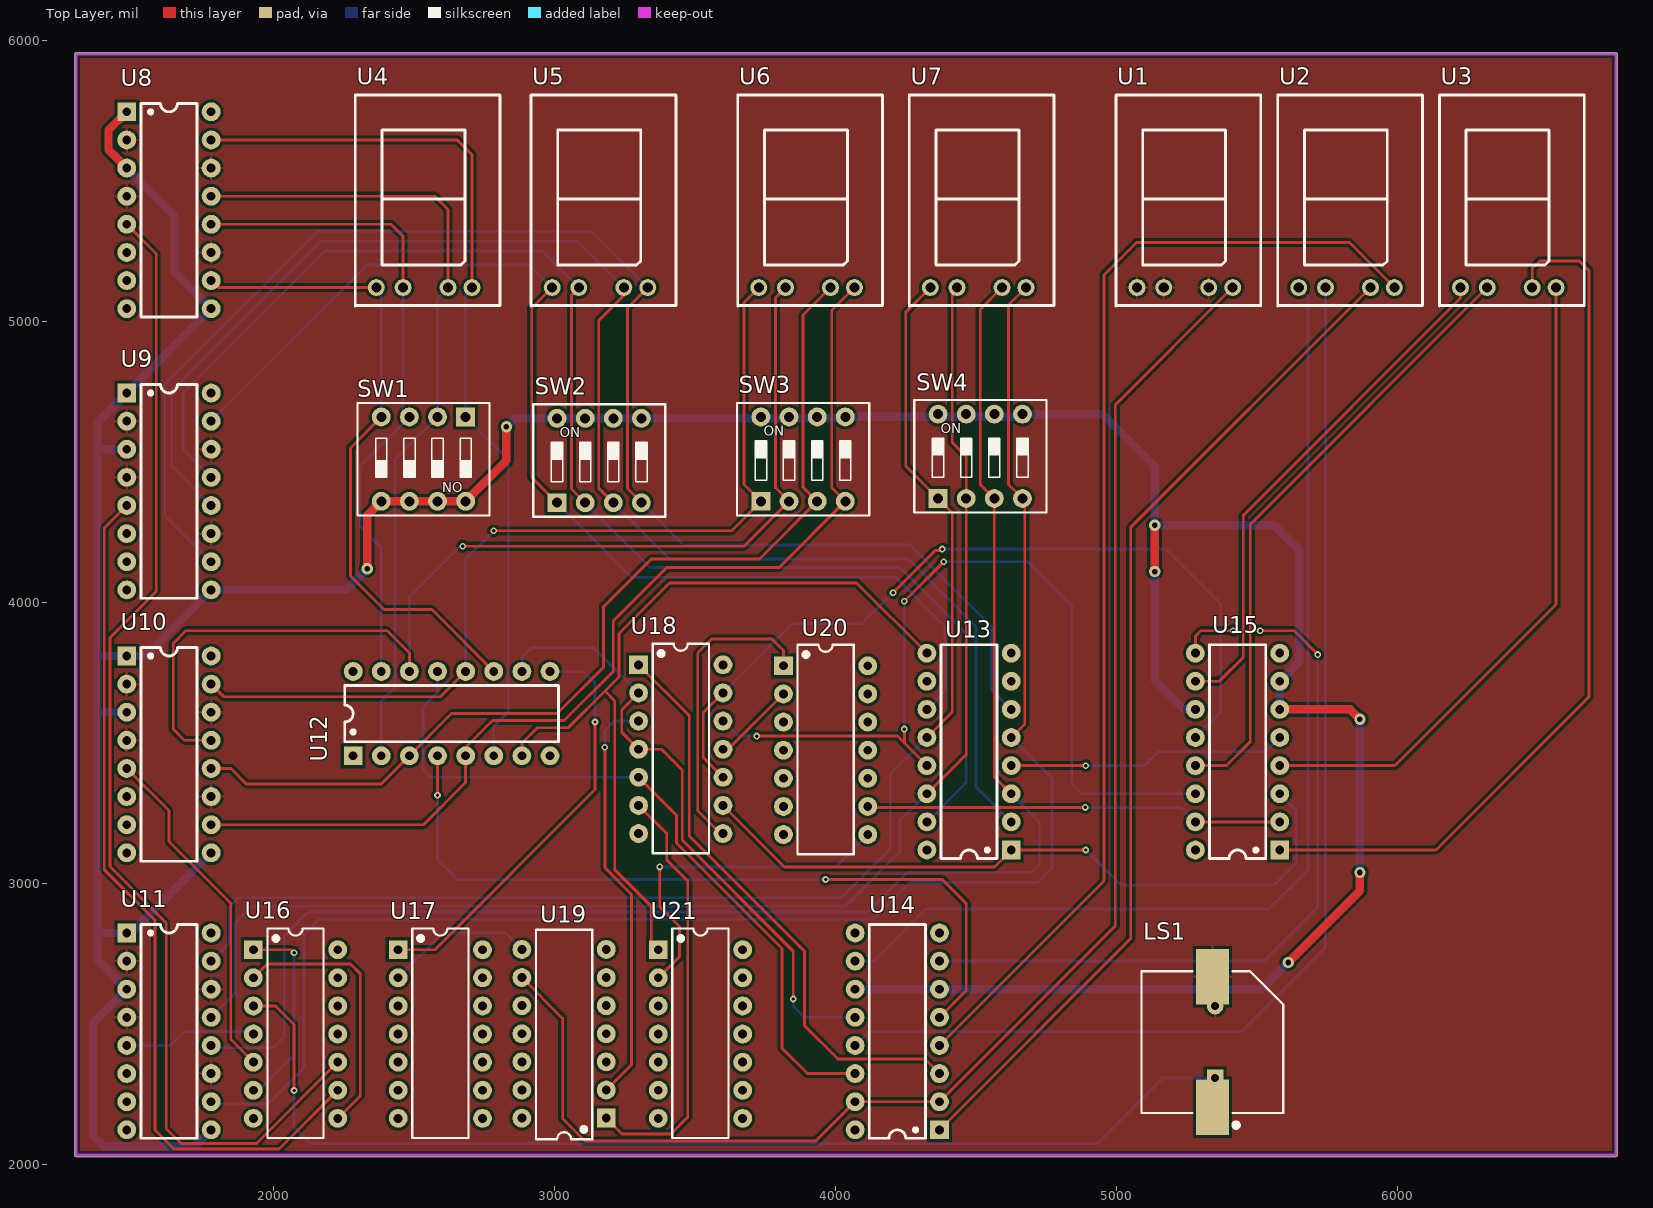
[diagram p0: Top Layer view]
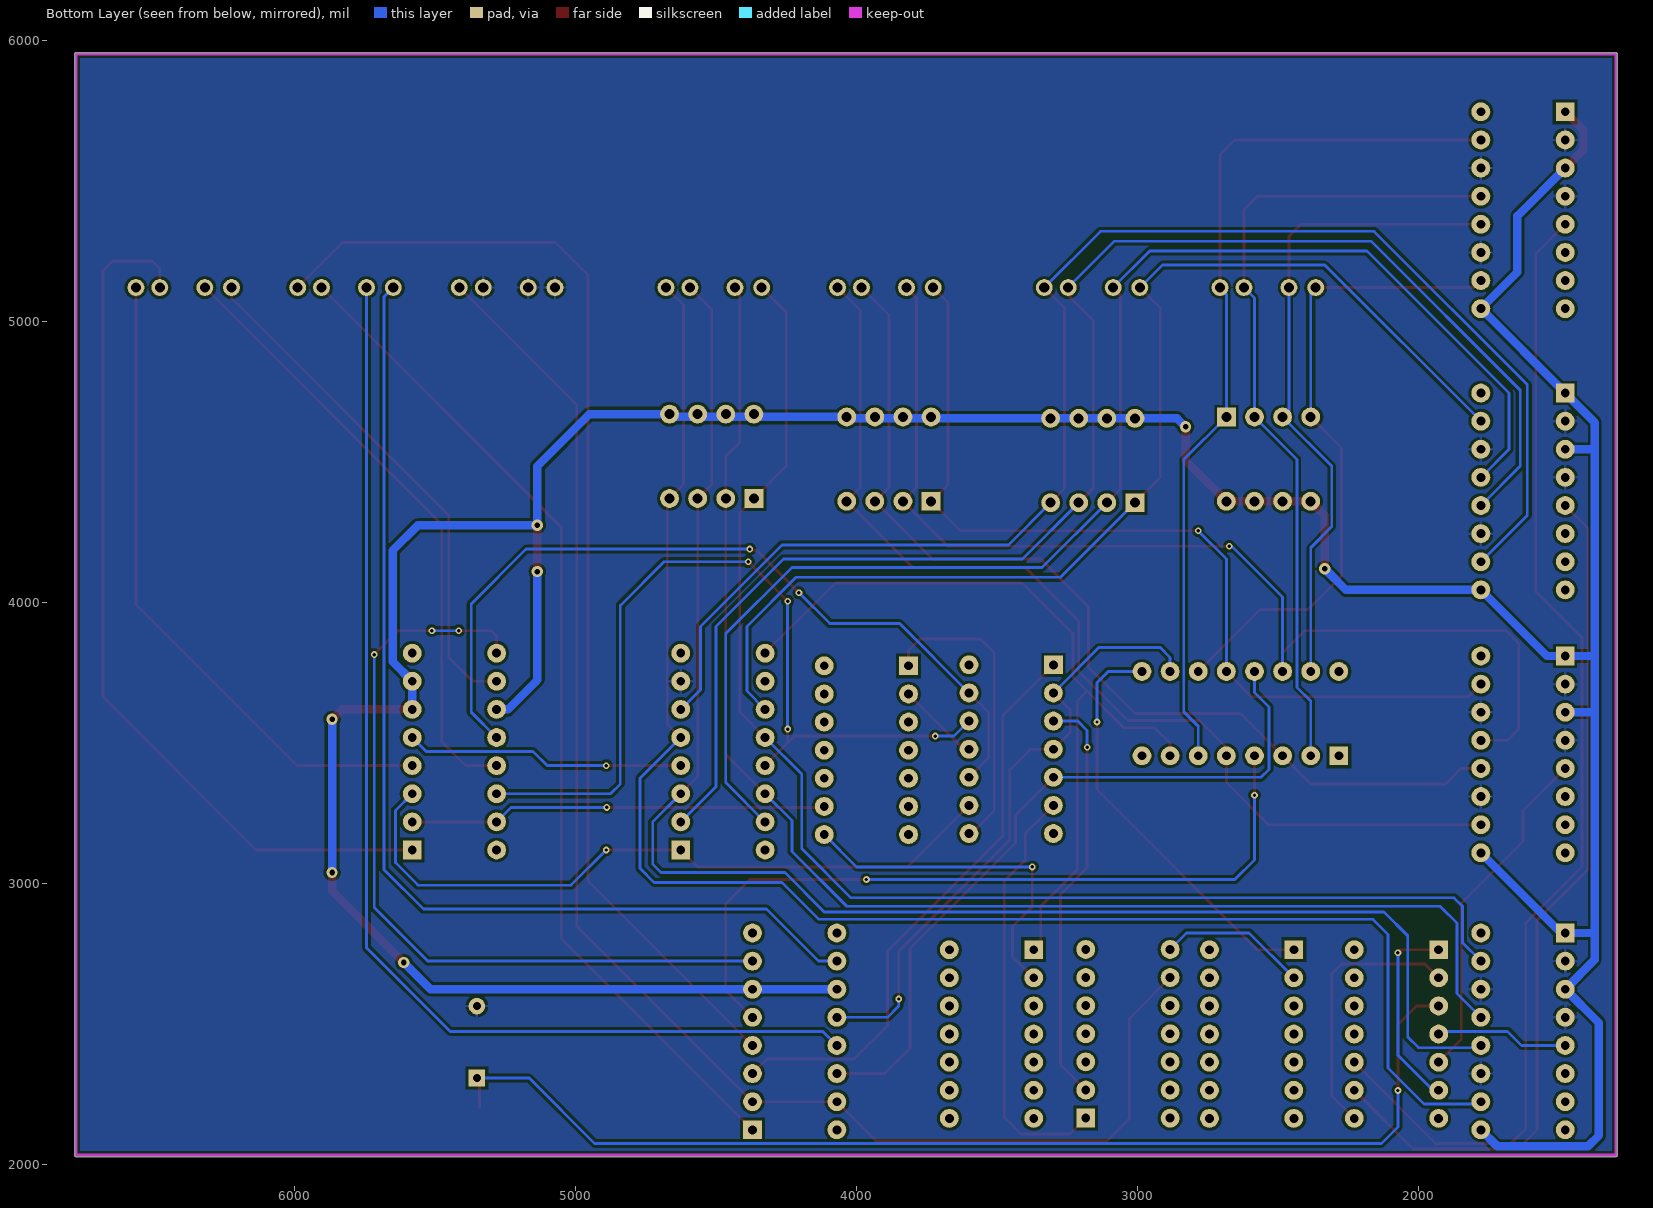
[diagram p1: Bottom Layer view, seen from below]
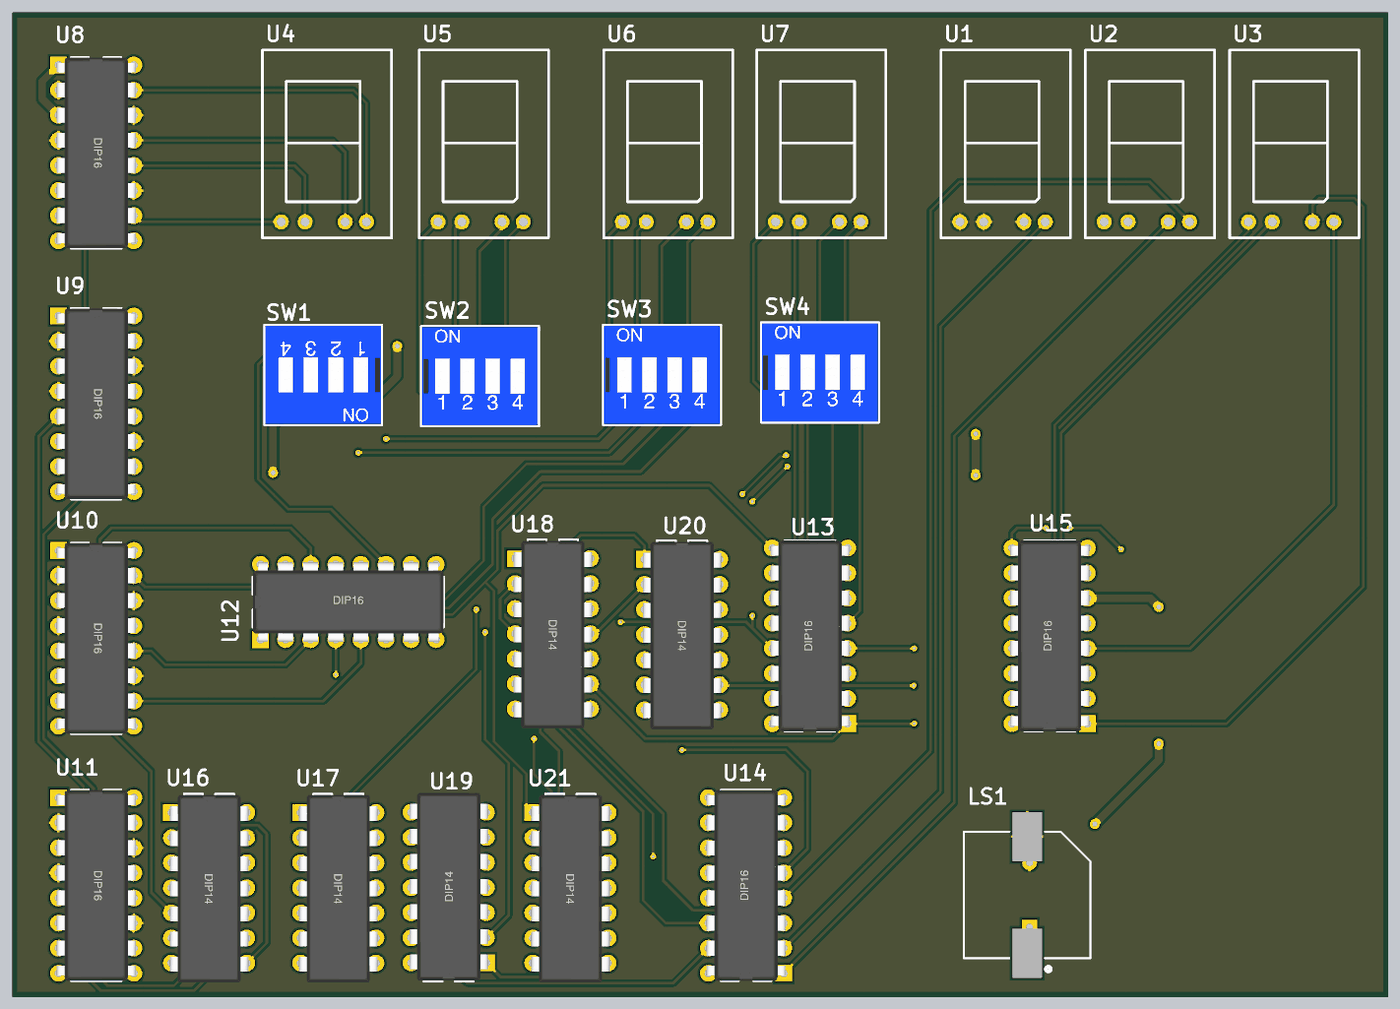
[diagram p2: 3D render of the assembled board from above, using the file's embedded part models]
# Altium PCB MISC62801.PcbDoc
Units mil, origin at the board's own origin, x right, y up, seen from the top; angles counter-clockwise.
Board outline 5485.03 x 3925.03 mil, 2 copper layers (Top Layer, Bottom Layer); 26 components, 52 nets, 276 pads, 29 vias.

## Layer stack, top to bottom (the 12.6 mil dielectric is the usual default, probably not edited)
Top Solder: solder mask 0.4, Solder Resist, Dk 3.5
Top Layer: signal copper 1.4
Dielectric 1: dielectric 12.6, FR-4, Dk 4.8
Bottom Layer: signal copper 1.4
Bottom Solder: solder mask 0.4, Solder Resist, Dk 3.5

## Board outline
1300,2029.98 cw(c1300,2035) 1294.98,2035 1294.98,5950 cw(c1300,5950) 1300,5955.02 6775,5955.02 cw(c6775,5950) 6780.02,5950 6780.02,2035 cw(c6775,2035) 6775,2029.98

## Design rules (kind name [scope] priority, off if disabled: settings)
Clearance [All] p1: gap=10
MinimumSolderMaskSliver [All] p1: minsoldermaskwidth=0
PolygonConnect [All] p1: connectstyle=Relief reliefconductorwidth=10 reliefentries=4 polygonreliefangle="90 Angle" airgapwidth=10
RoutingVias [All] p1: holewidth=28 width=50 viastyle="Through Hole" minholewidth=28 minwidth=50 maxholewidth=28 maxwidth=50
SilkToSilkClearance [All] p1: silktosilkclearance=0
SilkToSolderMaskClearance [IsPad] p1: minsilkscreentomaskgap=0 clearancetoexposedcopper=TRUE
SolderMaskExpansion [All] p1: expansion=4
Width [All] p1: maxlimit=13110.24 minlimit=10 preferedwidth=10
27 further rules are at their usual default settings.

## Components (designator, comment, footprint, x,y, rotation, side; value= is the part's Value field where it differs from the comment)
LS1 "Buzzer" ABSM-1574 5340.55,2204.76 r90 top
SW1 "SW-4P" "CSW DIP-4P" 2535,4510 r180 top
SW2 "SW-4P" "CSW DIP-4P" 3160,4505 r0 top
SW3 "SW-4P" "CSW DIP-4P" 3885,4510 r0 top
SW4 "SW-4P" "CSW DIP-4P" 4515,4520 r0 top
U1 "LCD1" DCD-HEX 5255,5430 r0 top
U2 "LCD1" DCD-HEX 5830,5430 r0 top
U3 "LCD1" DCD-HEX 6405,5430 r0 top
U4 "LCD1" DCD-HEX 2550,5430 r0 top
U5 "LCD1" DCD-HEX 3175,5430 r0 top
U6 "LCD1" DCD-HEX 3910,5430 r0 top
U7 "LCD1" DCD-HEX 4520,5430 r0 top
U8 "SN74LS85N" DIP16 1630,5395 r0 top
U9 "SN74LS85N" DIP16 1630,4395 r0 top
U10 "SN74LS85N" DIP16 1630,3460 r0 top
U11 "SN74LS85N" DIP16 1630,2475 r0 top
U12 "74HC283D" DIP16 2635,3605 r90 top
U13 "74HC283D" DIP16 4475,3470 r180 top
U14 "74HC283D" DIP16 4220,2475 r180 top
U15 "74HC283D" DIP16 5430,3470 r180 top
U16 "74LS32" DIP14 2080,2465.57 r0 top
U17 "74LS04" DIP14 2595,2465.57 r0 top
U18 "74LS00" DIP14 3450,3478.53 r0 top
U19 "MC14023UBCL" DIP14 3035,2466.47 r180 top
U20 "MC14023UBCL" DIP14 3965,3475 r0 top
U21 "74LS04" DIP14 3520,2465.57 r0 top

## Footprints (in the part's own frame and the unit in brackets; to place one, negate y for a bottom-side part, rotate by r counter-clockwise, add the part's x,y. Pads: shape width x height; smd on the part's side, far side on the other; paste and mask are expansions set on the pad)
ABSM-1574 [mm] "Magnetic Transducer Buzzer"
  rect 5x3 smd: 1(0,0) 2(11.8,0)
  rect 1.5x1.5 hole 0.7: 1A(2.65,-0.24)
  round 1.5 hole 0.7: 2A(9.15,-0.24)
  silkscreen extent -1.83,-6.4 12.3,6.4
"CSW DIP-4P" [mm] "11.7*9.9*7mm"
  rect 1.7x1.7 hole 0.9: 1(-3.81,-3.81)
  round 1.7 hole 0.9: 2(-1.27,-3.81) 3(1.27,-3.81) 4(3.81,-3.81) 5(3.81,3.81) 6(1.27,3.81) 7(-1.27,3.81) 8(-3.81,3.81)
  silkscreen extent -5.97,-5.08 5.97,5.08, body extent -5.86,-4.95 5.86,4.95, height 6.65
DCD-HEX [mil]
  round 60 hole 36 paste+0 mask+2: 1(-182.5,-310) 2(-87.5,-310)
  round 60 hole 36 paste+0 mask+4: 3(72.5,-310) 4(157.5,-310)
  silkscreen extent -258,-375 258,375
DIP14 [mm]
  rect 1.7x1.7 hole 0.8: 1(-3.81,7.62)
  round 1.7 hole 0.8: 2(-3.81,5.08) 3(-3.81,2.54) 4(-3.81,0) 5(-3.81,-2.54) 6(-3.81,-5.08) 7(-3.81,-7.62) 8(3.81,-7.62) 9(3.81,-5.08) 10(3.81,-2.54) 11(3.81,0) 12(3.81,2.54) 13(3.81,5.08) 14(3.81,7.62)
  silkscreen extent -2.54,-9.4 2.54,9.53, body extent -3.98,-9.6 3.98,9.4, height 4.1
DIP16 [mm]
  rect 1.7x1.7 hole 0.8: 1(-3.81,8.89)
  round 1.7 hole 0.8: 2(-3.81,6.35) 3(-3.81,3.81) 4(-3.81,1.27) 5(-3.81,-1.27) 6(-3.81,-3.81) 7(-3.81,-6.35) 8(-3.81,-8.89) 9(3.81,-8.89) 10(3.81,-6.35) 11(3.81,-3.81) 12(3.81,-1.27) 13(3.81,1.27) 14(3.81,3.81) 15(3.81,6.35) 16(3.81,8.89)
  silkscreen extent -2.54,-9.65 2.54,9.65, body extent -4.02,-9.65 4.02,9.65, height 4.45

## Part data
LS1: "Magnetic Transducer Buzzer"
SW1 SW2 SW3 SW4: "4-way coded switch"
U12 U13 U14 U15: library part HD74HC283RP
U16: "Quad 2-input OR gate"
U17 U21: "Hex inverter"
U18: "Quad 2-input NAND gate"

## Via types
v1: diameter 24, hole 12, Top Layer to Bottom Layer, 22 vias
v2: diameter 40, hole 20, Top Layer to Bottom Layer, 7 vias

## Nets (pads, with @x,y where several pads share a name; then routed paths per layer and width w, separated by ;. In a path a pad name is that pad's centre, name@x,y a point inside that pad or via, vN(x,y) a via of type N, cw(c..) or ccw(c..) an arc to the next point about the centre after c; other vN are vias at no path point)
+5: SW1.5 SW1.6 SW1.7 SW1.8 SW2.5 SW2.6 SW2.7 SW2.8 SW3.5 SW3.6 SW3.7 SW3.8 SW4.5 SW4.6 SW4.7 SW4.8 U8.1 U8.3 U8.9 U9.1 U9.3 U9.9 U10.1 U10.3 U10.9 U11.1 U11.3 U11.9 U14.6 U14.11 U15.6 U15.7 U15.11 | length 14597.2
  Top Layer w30: U8.3 1415,5610 1415,5680 U8.1 ; v2(2335,4120) 2335,4310 SW1.5 SW1.6 SW1.7 SW1.8 2830,4505 v2(2830,4625) ; v2(5135,4110) v2(5135,4275) ; U15.6 5830,3620 v2(5865,3585) ; v2(5610,2720) 5865,2975 v2(5865,3040)
  Bottom Layer w30: U10.3 1380,3610 1375,3605 ; U9.3 1375,4545 ; U8.3 1650,5375 1650,5175 U8.9 U9.1 1375,4640 1375,4545 ; U11.9 1721.54,2066.54 1398.46,2066.54 1360,2105 1360,2505 U11.3 1375,2730 1375,2835 ; U10.9 1495,2825 U11.1 1385,2825 1375,2835 ; v2(2335,4120) 2260,4045 U9.9 1545,3810 U10.1 1375,3810 ; v2(2830,4625) 2860,4655 SW2.8 SW2.7 SW2.6 SW2.5 4030,4655 SW3.5 4655,4660 SW4.5 4950,4670 5135,4485 v2(5135,4275) 5560,4275 5650,4185 5650,3790 U15.7 U15.6 ; U14.11 U14.6 5515,2625 v2(5610,2720) ; v2(5135,4110) 5135,3725 5240,3620 U15.11 ; v2(5865,3040) v2(5865,3585) ; 1375,2835 1375,3605 ; 1375,3605 1375,3810 ; 1375,3810 1375,4545
GND: LS1.2 LS1.2A U1.1 U1.2 U1.3 U8.2 U8.4 U8.11 U8.14 U9.2 U9.4 U9.11 U9.14 U10.2 U10.4 U10.11 U10.14 U11.2 U11.4 U11.11 U11.14 U13.7
NetLS1_1: LS1.1 LS1.1A U16.3 | length 4040.9
  Top Layer w10: U16.3 2009.43,2565.57 2075,2500 v1(2075,2265) ; LS1.1 5340.55,2299.65 LS1.1A
  Bottom Layer w10: v1(2075,2265) 2075,2135 2133.46,2076.54 4931.54,2076.54 5164.09,2309.09 LS1.1A
NetSW1_1: SW1.1 U4.4 U8.15 U12.6 | length 3180.2
  Top Layer w10: U8.15 2655,5645 2707.5,5592.5 U4.4
  Bottom Layer w10: U4.4 2685,5097.5 SW1.1 2836.54,4508.46 2836.54,3611.54 2785,3560 U12.6
NetSW1_2: SW1.2 U4.3 U8.13 U12.2 | length 2903.1
  Top Layer w10: U8.13 2575,5445 2622.5,5397.5 U4.3
  Bottom Layer w10: U12.2 2385,3650 2433.46,3698.46 2433.46,4508.46 SW1.2 2585,5082.5 U4.3
NetSW1_3: SW1.3 U4.2 U8.12 U12.15 | length 2360.5
  Top Layer w10: U8.12 2420,5345 2462.5,5302.5 U4.2
  Bottom Layer w10: U12.15 2385,4195 2310,4270 2310,4485 SW1.3 2462.5,4682.5 U4.2
NetSW1_4: SW1.4 U4.1 U8.10 U12.11 | length 2351.2
  Top Layer w10: U8.10 1805,5120 U4.1 U4.1@2385,5102.5 ; SW1.4 2275,4550 2275,4095 2395,3975 2565,3975 U12.11
  Bottom Layer w10: U4.1 2385,5102.5 SW1.4
NetSW2_1: SW2.1 U5.1 U9.15 U13.11 | length 4192
  Top Layer w10: U5.1 2920,5047.5 2920,4445 SW2.1
  Bottom Layer w10: U9.15 2335,5200 2912.5,5200 U5.1 ; SW2.1 3275,4090 4215,4090 4390,3915 4390,3685 U13.11
NetSW2_2: SW2.2 U5.2 U9.13 U13.15 | length 5083.4
  Top Layer w10: U5.2 3061.54,5094.04 3061.54,4403.46 SW2.2
  Bottom Layer w10: U9.13 1680,4545 1680,4745 2185,5250 2957.5,5250 U5.2 ; SW2.2 3340,4125 4230,4125 4465,3890 4465,3360 U13.15
NetSW2_3: SW2.3 U5.3 U9.12 U13.2 | length 5405.6
  Top Layer w10: SW2.3 3158.46,4406.54 3158.46,5003.46 3247.5,5092.5 U5.3
  Bottom Layer w10: U9.12 1640,4485 1640,4755 2170,5285 3082.5,5285 U5.3 ; SW2.3 3410,4155 4260,4155 4500,3915 4500,3345 U13.2
NetSW2_4: SW2.4 U5.4 U9.10 U13.6 | length 5316.5
  Top Layer w10: SW2.4 3260,4405 3260,5047.5 U5.4
  Bottom Layer w10: U9.10 1615,4310 1615,4775 2160,5320 3132.5,5320 U5.4 ; SW2.4 3460,4205 4265,4205 4555,3915 4555,3690 U13.6 U13.6@4625,3645.11
NetSW3_1: SW3.1 U6.1 U10.15 U12.12 | length 3302.4
  Top Layer w10: U10.15 1825,3665 2595,3665 U12.12 ; v1(2785,4255) 3630,4255 SW3.1 3675,4420 3675,5067.5 U6.1
  Bottom Layer w10: U12.12 2685,4155 v1(2785,4255)
NetSW3_2: SW3.2 U6.2 U10.13 U12.14 | length 3968.3
  Top Layer w10: U10.13 1685,3510 1645,3550 1645,3855 1690,3900 2405,3900 2485,3820 U12.14 ; v1(2675,4200) 3675,4200 SW3.2 3786.54,4408.46 3786.54,5084.04 U6.2
  Bottom Layer w10: U12.14 2485,4020 2670,4205 v1(2675,4200)
NetSW3_3: SW3.3 U6.3 U10.12 U12.3 | length 3541.1
  Top Layer w10: U10.12 1850,3410 1905,3355 2385,3355 U12.3 2635,3605 3010,3605 3175,3770 3175,3985 3345,4155 3730,4155 SW3.3 3885,4410 3885,5022.5 U6.3
NetSW3_4: SW3.4 U6.4 U10.10 U12.5 | length 3723.6
  Top Layer w10: U10.10 2535,3210 2685,3360 U12.5 2685,3485 2780,3580 3035,3580 3210,3755 3210,3935 3400,4125 3800,4125 SW3.4 3986.54,4408.46 3986.54,5039.04 U6.4
NetSW4_1: SW4.1 U7.1 U11.15 U13.12 | length 4847.6
  Top Layer w10: U13.12 4415,3610 4415,4320 SW4.1 4250,4485 4250,5032.5 U7.1
  Bottom Layer w10: U11.15 1845,2790 1845,2920 1875,2950 4020,2950 4195,3125 4195,3390 U13.12
NetSW4_2: SW4.2 U7.2 U11.13 U13.14 | length 4971.1
  Top Layer w10: U13.14 4465,3460 SW4.2 4465,4520 4415,4570 4415,5102.5 U7.2
  Bottom Layer w10: U11.13 1865,2610 1865,2860 1925,2920 4035,2920 4230,3115 4230,3225 U13.14
NetSW4_3: SW4.3 U7.3 U11.12 U13.3 | length 5603.3
  Top Layer w10: U7.3 4515,5042.5 4515,4420 SW4.3 4565,3380 U13.3
  Bottom Layer w10: U11.12 1780,2417.1 2002.1,2417.1 2040,2455 2040,2815 2125,2900 4115,2900 4255,3040 4695,3040 4725,3070 4725,3220 U13.3
NetSW4_4: SW4.4 U7.4 U11.10 U13.5 | length 5818.5
  Top Layer w10: U13.5 4673.46,3568.46 4673.46,4361.54 SW4.4 4615,4420 4615,5057.5 U7.4
  Bottom Layer w10: U11.10 1780,2217.1 1982.1,2217.1 2110,2345 2110,2820 2163.46,2873.46 4133.46,2873.46 4265,3005 4720,3005 4770,3055 4770,3375 U13.5
NetU1_4: U1.4 U14.2 U14.15 U19.9 | length 5319.5
  Top Layer w10: U19.9 3030,2521.47 3030,2165 3110,2085 3930,2085 U14.15 U14.2 4995,2850 4995,4702.5 U1.4
NetU2_1: U2.1 U14.10 | length 3828.1
  Bottom Layer w10: U14.10 4135,2725 4320,2910 5540,2910 5680,3050 5680,5087.5 U2.1
NetU2_2: U2.2 U14.13 | length 4163.9
  Bottom Layer w10: U14.13 4120,2475 5445,2475 5742.5,2772.5 U2.2
NetU2_3: U2.3 U14.1 | length 3629.8
  Top Layer w10: U14.1 5050,2805 5050,4267.5 U2.3
NetU2_4: U2.4 U14.4 | length 4128.7
  Top Layer w10: U14.4 4955,3010 4955,5165 5070,5280 5827.5,5280 U2.4
NetU3_1: U3.1 U15.10 | length 1840.2
  Top Layer w10: U15.10 5365,3720 5450,3805 5450,4310 6222.5,5082.5 U3.1
NetU3_2: U3.2 U15.13 | length 2194.2
  Top Layer w10: U15.13 5390,3420 5475,3505 5475,4277.5 U3.2
NetU3_3: U3.3 U15.1 | length 3136.6
  Top Layer w10: U15.1 6135,3120 6680,3665 6680,5180 6645,5215 6505,5215 6477.5,5187.5 U3.3
NetU3_4: U3.4 U15.4 | length 2347.1
  Top Layer w10: U15.4 5990,3420 6562.5,3992.5 U3.4
NetU8_5: U8.5 U16.10 | length 4161.5
  Top Layer w10: U8.5 1585,5240 1585,4040 1420,3875 1420,3061.54 1620,2861.54 1620,2130 1673.46,2076.54 1940.97,2076.54 U16.10
NetU9_5: U9.5 U16.9 | length 3092.6
  Top Layer w10: U9.5 1400,4265 1400,3050 1580,2870 1580,2125 1648.46,2056.54 2020.97,2056.54 U16.9
NetU10_5: U10.5 U16.5 | length 1230.8
  Top Layer w10: U10.5 1630,3260 1630,3150 1850,2930 1850,2445.57 U16.5
NetU11_5: U11.5 U16.4 | length 474.6
  Bottom Layer w10: U11.5 1635,2425 1685,2475 1920.57,2475 U16.4
NetU12_4: U12.4 U14.5 | length 2758.6
  Top Layer w10: v1(2585,3315) U12.4 ; v1(3965,3015) 4380,3015 4465,2930 4465,2620 U14.5
  Bottom Layer w10: v1(2585,3315) 2585,3085 2655,3015 v1(3965,3015)
NetU12_7: U12.7 U13.9 U21.1 | length 2913.6
  Top Layer w10: U12.7 2885,3500 2940,3555 3050,3555 3180,3685 ; U21.1 3345,2790.57 3345,2920 3215,3050 3215,3650 3180,3685 ; U13.9 4075,4070 3410,4070 3230,3890 3230,3735 3180,3685
NetU12_9: U12.9 U17.1 | length 1492.4
  Top Layer w10: U17.1 2575.57,2765.57 3145,3335 v1(3145,3575)
  Bottom Layer w10: U12.9 3105,3755 3145,3715 v1(3145,3575)
NetU12_10: U12.10 U14.12 U18.2 U18.4 | length 2221.7
  Top Layer w10: U18.2 3240,3618.53 3240,3538.53 U18.4 3381.47,3478.53 3455,3405 3455,3155 3850,2760 v1(3850,2590)
  Bottom Layer w10: U12.10 2885,3805 2920,3840 3138.53,3840 U18.2 ; v1(3850,2590) 3850,2565 3890,2525 U14.12
NetU12_13: U12.13 U14.14 U18.5 | length 2620
  Top Layer w10: U18.5 3435,3243.53 3435,3145 3810,2770 3810,2415 3900,2325 U14.14
  Bottom Layer w10: U12.13 2585,3680 2533.46,3628.46 2533.46,3406.54 2561.47,3378.53 U18.5
NetU13_1: U13.1 U15.3 U18.9 | length 2510.1
  Top Layer w10: U18.9 3818.53,3060 4565,3060 U13.1 v1(4890,3120)
  Bottom Layer w10: v1(4890,3120) 5015,2995 5560,2995 5640,3075 5640,3260 U15.3
NetU13_4: U13.4 U15.5 | length 996.4
  Top Layer w10: U13.4 v1(4890,3420)
  Bottom Layer w10: v1(4890,3420) 5100,3420 5150,3470 5530,3470 U15.5
NetU13_13: U13.13 U15.14 U18.12 | length 3102.4
  Top Layer w10: v1(3720,3525) 4220,3525 4245,3500 ; v1(4245,3550) 4245,3500 ; v1(4245,4005) v1(4385,4145) ; U13.13 4245,3500
  Bottom Layer w10: U18.12 3653.53,3525 v1(3720,3525) ; v1(4245,3550) v1(4245,4005) ; v1(4385,4145) 4685,4145 4840,3990 4840,3355 4875,3320 U15.14
NetU14_3: U14.3 U18.1 | length 2078.3
  Top Layer w10: U18.1 3480,3598.53 3480,3170 3890,2760 3890,2495 4008.46,2376.54 4318.46,2376.54 U14.3
NetU14_7: U14.7 U15.9 | length 2867.2
  Top Layer w10: U15.9 5280,3880 5300,3900 v1(5415,3900) ; v1(5510,3900) 5630,3900 v1(5715,3815)
  Bottom Layer w10: U14.7 5525,2725 5715,2915 v1(5715,3815) v1@5710,3815 ; v1(5415,3900) v1(5510,3900)
NetU15_2: U15.2 U15.15 U20.9 | length 1489.8
  Top Layer w10: U20.9 4115,3271.54 v1(4888.46,3271.54) ; U15.15 U15.2
  Bottom Layer w10: v1(4888.46,3271.54) 5228.46,3271.54 U15.15
NetU15_12: U15.12 U18.10 U18.13 | length 2925.8
  Top Layer w10: U18.10 3530,3448.53 3530,3608.53 U18.13 ; v1(4205,4035) 4355,4185 v1@4375,4185
  Bottom Layer w10: U18.13 3846.47,3925 4095,3925 v1(4205,4035) ; v1(4380,4190) 5175,4190 5370,3995 5370,3610 U15.12
NetU16_1: U16.1 U16.6 | length 710.9
  Top Layer w10: U16.1 2064.43,2765.57 v1(2075,2755)
  Bottom Layer w10: U16.6 1950.57,2265.57 2075,2390 v1(2075,2755)
NetU16_2: U16.2 U16.8 | length 962.5
  Top Layer w10: U16.2 1979.43,2715 2275,2715 2310,2680 2310,2245.57 U16.8
NetU17_2: U17.2 U19.8 | length 530.3
  Bottom Layer w10: U17.2 2604.43,2825 2826.47,2825 U19.8
NetU18_3: U18.3 U19.2 | length 1489
  Top Layer w10: v1(3180,3485) 3180,3056.72 3275,2961.72 3275,2356.47 U19.2
  Bottom Layer w10: v1(3180,3485) 3180,3545 3213.53,3578.53 U18.3
NetU18_6: U18.6 U19.1 | length 1519.3
  Top Layer w10: U19.1 3241.47,2110 3415,2110 3475,2170 3475,3010 3400,3085 3400,3178.53 U18.6
NetU18_8: U18.8 U20.1 | length 1081
  Top Layer w10: U18.8 3591.47,3178.53 3510,3260 3510,3820 3560,3870 3775,3870 3815,3830 U20.1
NetU18_11: U18.11 U20.2 | length 296.4
  Top Layer w10: U18.11 3618.53,3478.53 U20.2
NetU20_8: U20.8 U21.2 | length 1242.1
  Top Layer w10: U21.2 3445,2740.57 3445,2848.28 3375,2918.28 v1(3375,3060)
  Bottom Layer w10: v1(3375,3060) 4000,3060 U20.8
pads on no net: U8.6 U8.7 U8.8 U8.16 U9.6 U9.7 U9.8 U9.16 U10.6 U10.7 U10.8 U10.16 U11.6 U11.7 U11.8 U11.16 U12.1 U12.8 U12.16 U13.8 U13.10 U13.16 U14.8 U14.9 U14.16 U15.8 U15.16 U16.7 U16.11 U16.12 U16.13 U16.14 U17.3 U17.4 U17.5 U17.6 U17.7 U17.8 U17.9 U17.10 U17.11 U17.12 U17.13 U17.14 U18.7 U18.14 U19.3 U19.4 U19.5 U19.6 U19.7 U19.10 U19.11 U19.12 U19.13 U19.14 U20.3 U20.4 U20.5 U20.6 U20.7 U20.10 U20.11 U20.12 U20.13 U20.14 U21.3 U21.4 U21.5 U21.6 U21.7 U21.8 U21.9 U21.10 U21.11 U21.12 U21.13 U21.14

## Polygon pours and split planes (outlines as drawn)
GND on Bottom Layer "G" (solid, remove dead copper, pour order 0): 965,6135 1095,6265 6835,6265 6835,1995 6905,1925 6735,1755 910,1755
GND on Top Layer "G" (solid, remove dead copper, pour order 4): 895,6120 1005,6230 7300,6230 7300,2075 6785,1560 6435,1210 685,1210

## Keep-outs
Keep-Out Layer:
  lines w10: 1450,5950 6775,5950 6775,2035 1300,2035 1300,5950 1475,5950